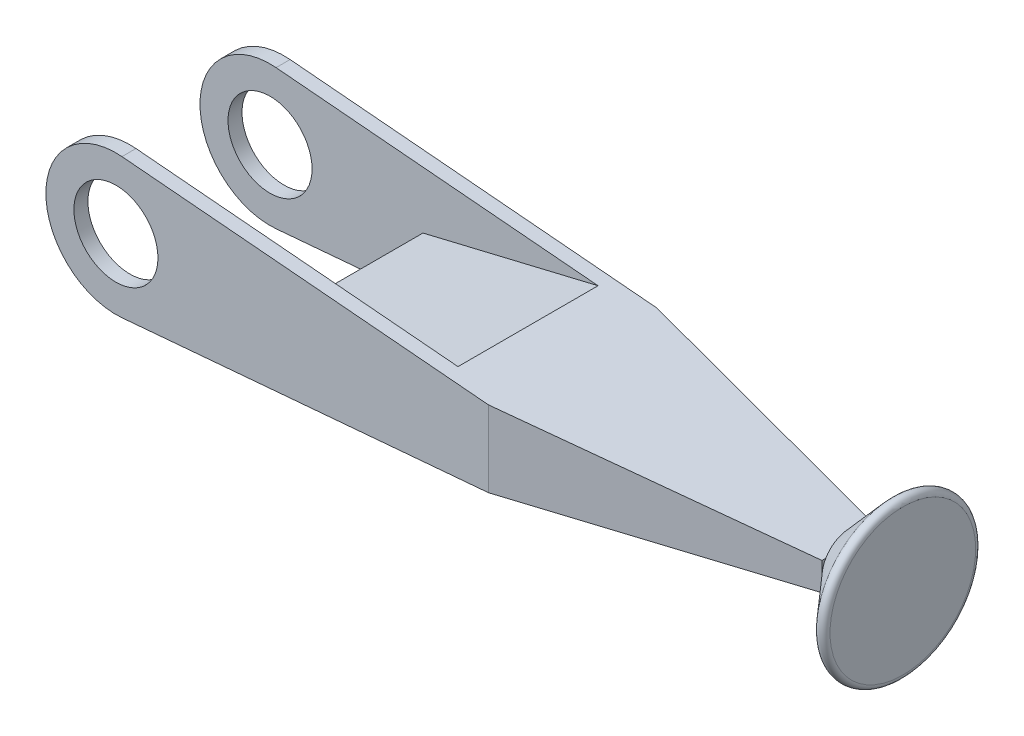
SolidWorks part; units mm, degrees
ref_plane "Front Plane" through (0, 0, 0) normal (0, 0, 1) x (1, 0, 0)
ref_plane "Top Plane" through (0, 0, 0) normal (0, 1, 0) x (1, 0, 0)
ref_plane "Right Plane" through (0, 0, 0) normal (1, 0, 0) x (0, 0, -1)
other "Configuration Table"
sketch "Sketch13" plane through (0, 0, 0) normal (0, 0, 1) x (1, 0, 0)
  line L0 (2.1572, 24.9068) -> (232, 5)
  line L1 (0, 0) -> (322.4267, 0) construction
  line L2 (232, 5) -> (232, -5)
  line L3 (2.1572, -24.9068) -> (232, -5)
  arc A0 (2.1572, 24.9068) -> (2.1572, -24.9068) centre (0, 0) ccw
  circle A1 centre (0, 0) radius 15
  point P8 (232, 0)
  dimension "D1" = 50
  dimension "D4" = 30
  dimension "D2" = 5
  dimension "D3" = 232
extrude "Boss-Extrude6" add sketch "Sketch13" along normal blind 5
sketch "Sketch14" plane through (0, 0, 5) normal (0, 0, 1) x (1, 0, 0)
  line L0 (232, 5) -> (117.0786, 14.9534)
  line L1 (232, 5) -> (2.1572, 24.9068) construction
  line L2 (117.0786, 14.9534) -> (54.5889, 0)
  line L3 (54.5889, 0) -> (117.0786, -14.9534)
  line L4 (2.1572, -24.9068) -> (232, -5) construction
  line L5 (117.0786, -14.9534) -> (232, -5)
  line L6 (232, -5) -> (232, 5) construction
  line L7 (232, -5) -> (232, 5)
extrude "Boss-Extrude7" add sketch "Sketch14" along normal blind 50
sketch "Sketch15" plane through (0, 0, 5) normal (0, 0, 1) x (1, 0, 0)
  line L4 (117.0786, -14.9534) -> (54.5889, 0)
  line L5 (54.5889, 0) -> (117.0786, 14.9534)
  line L6 (117.0786, 14.9534) -> (2.1572, 24.9068)
  line L7 (2.1572, -24.9068) -> (117.0786, -14.9534)
  line L10 (117.0786, 14.9534) -> (2.1572, 24.9068)
  line L11 (2.1572, -24.9068) -> (117.0786, -14.9534)
  line L13 (232, -5) -> (232, 5)
  line L14 (232, 5) -> (117.0786, 14.9534)
  line L15 (117.0786, 14.9534) -> (54.5889, 0)
  line L16 (54.5889, 0) -> (117.0786, -14.9534)
  line L17 (117.0786, -14.9534) -> (232, -5)
  line L18 (232, -5) -> (232, 5)
  line L19 (232, 5) -> (117.0786, 14.9534)
  line L22 (117.0786, -14.9534) -> (232, -5)
  circle A0 centre (0, 0) radius 15 construction
  arc A1 (2.1572, 24.9068) -> (2.1572, -24.9068) centre (0, 0) ccw
  arc A2 (2.1572, 24.9068) -> (2.1572, -24.9068) centre (0, 0) ccw
  circle A3 centre (0, 0) radius 15
  dimension "D1" = 0
  dimension "D2" = 0
extrude "Boss-Extrude8" add sketch "Sketch15" along normal blind 5 from offset 50
sketch "Sketch16" plane through (0, 0, 0) normal (0, 1, 0) x (1, 0, 0)
  line L0 (54.5889, -30) -> (277.475, -30) construction
  line L1 (54.5889, -55) -> (54.5889, -5) construction
  line L2 (232, 0) -> (133.0118, 0)
  line L3 (232, 0) -> (2.1572, 0) construction
  line L4 (133.0118, 0) -> (232, -20)
  line L5 (232, -60) -> (232, 0) construction
  line L6 (232, -20) -> (232, 0)
  line L7 (232, -40) -> (232, -60)
  line L8 (232, -60) -> (133.0118, -60)
  line L10 (133.0118, -60) -> (232, -40)
  dimension "D1" = 10
extrude "Cut-Extrude2" cut sketch "Sketch16" against normal mid plane 83
sketch "Sketch20" plane through (0, 0, 0) normal (0, 1, 0) x (1, 0, 0)
  line L0 (232, -30) -> (232, -20)
  line L1 (232, -40) -> (232, -20) construction
  line L2 (232, -20) -> (250.8525, 1.266)
  line L3 (250.8525, 1.266) -> (250.8525, -30)
  line L4 (250.8525, -30) -> (232, -30)
revolve "Revolve4" add sketch "Sketch20" angle 360 about L4
fillet "Fillet2" radius 2 1 edges at (250.8525, 0, -1.266)
